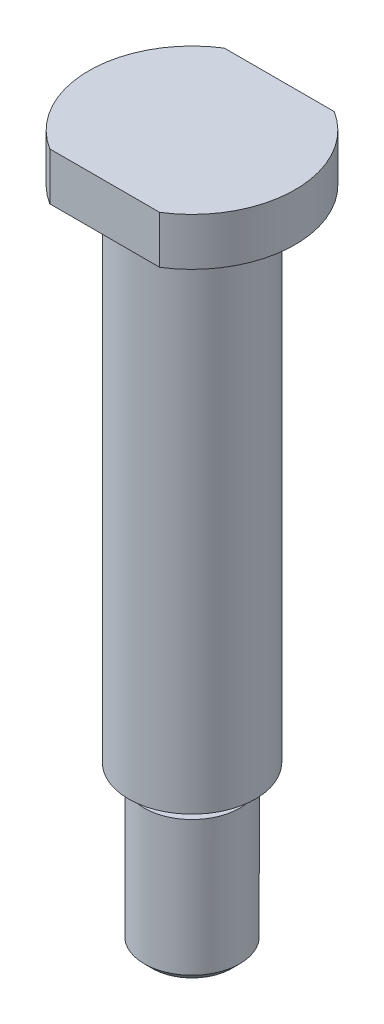
from build123d import *

# Parameters (mm, degrees)
SKETCH_1_R           = 4
EXTRUDE_1_DEPTH      = 31.5
SKETCH_2_R           = 3
EXTRUDE_2_DEPTH      = 10
SKETCH_3_R           = 6.5
EXTRUDE_3_DEPTH      = 3
SKETCH_4_OUTSIDE_W   = 24.63
SKETCH_4_OUTSIDE_H   = 24.63
SKETCH_4_OUTSIDE_W_2 = 13
SKETCH_4_OUTSIDE_H_2 = 11
CUT_EXTRUDE_1_DEPTH  = 46.439520244
CHAMFER_1_SIZE       = 0.5
SKETCH_5_W           = 0.5
SKETCH_5_H           = 1


with BuildPart() as part:
    # 草图1 → 凸台-拉伸1 (new body)
    with BuildSketch(Plane(origin=(0, 0, 0), x_dir=(1, 0, 0), z_dir=(0, 1, 0))):
        with Locations(Location((0, 0, 0), (0, 0, 270))):
            Circle(SKETCH_1_R)
    extrude(amount=EXTRUDE_1_DEPTH)

    # 草图2 → 凸台-拉伸2 (add)
    with BuildSketch(Plane.XZ):
        with Locations(Location((0, 0, 0), (0, 0, 270))):
            Circle(SKETCH_2_R)
    extrude(amount=EXTRUDE_2_DEPTH)

    # 草图3 → 凸台-拉伸3 (add)
    with BuildSketch(Plane(origin=(0, 31.5, 0), x_dir=(1, 0, 0), z_dir=(0, 1, 0))):
        with Locations(Location((0, 0, 0), (0, 0, 270))):
            Circle(SKETCH_3_R)
    extrude(amount=EXTRUDE_3_DEPTH)

    # 草图4 outside → 切除-拉伸1 (cut, through all)
    with BuildSketch(Plane(origin=(0, 34.5, 0), x_dir=(1, 0, 0), z_dir=(0, 1, 0))):
        Rectangle(SKETCH_4_OUTSIDE_W, SKETCH_4_OUTSIDE_H)
        Rectangle(SKETCH_4_OUTSIDE_W_2, SKETCH_4_OUTSIDE_H_2, mode=Mode.SUBTRACT)
    extrude(amount=-CUT_EXTRUDE_1_DEPTH, mode=Mode.SUBTRACT)

    # 倒角1
    chamfer_1_edges = [part.edges().sort_by_distance(p)[0] for p in [
        (0, -10, 3),
    ]]
    chamfer(chamfer_1_edges, length=CHAMFER_1_SIZE)

    # 草图5 → 切除-旋转1 (revolve, cut)
    with BuildSketch(Plane.XY, mode=Mode.PRIVATE) as cut_revolve_1_sk:
        with Locations((-2.75, -0.5)):
            Rectangle(SKETCH_5_W, SKETCH_5_H)
    revolve(cut_revolve_1_sk.sketch.rotate(Axis((0, 0, 0), (0, -1, 0)), 270), axis=Axis((0, 0, 0), (0, -1, 0)), mode=Mode.SUBTRACT)


solid = part.part
